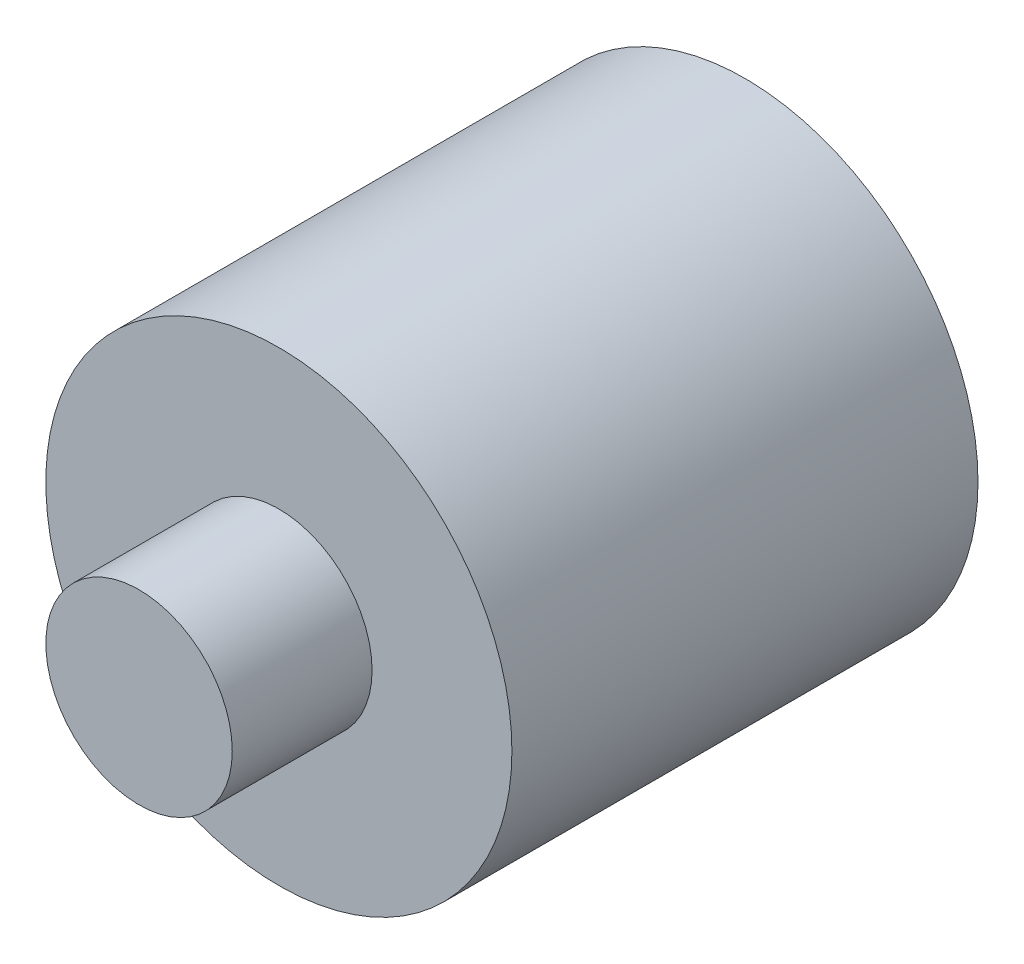
SolidWorks part; units mm, degrees
ref_plane "Front Plane" through (0, 0, 0) normal (0, 0, 1) x (1, 0, 0)
ref_plane "Top Plane" through (0, 0, 0) normal (0, 1, 0) x (1, 0, 0)
ref_plane "Right Plane" through (0, 0, 0) normal (1, 0, 0) x (0, 0, -1)
other "Configuration Table"
sketch "Sketch1" plane through (0, 0, 0) normal (0, 0, 1) x (1, 0, 0)
  circle A0 centre (0, 0) radius 2.5
  dimension "D1" = 5
extrude "Boss-Extrude1" add sketch "Sketch1" along normal blind 5
sketch "Sketch2" plane through (0, 0, 5) normal (0, 0, 1) x (1, 0, 0)
  circle A0 centre (0, 0) radius 1
  dimension "D1" = 2
extrude "Boss-Extrude2" add sketch "Sketch2" along normal blind 1.5
sketch "Sketch3" plane through (0, 0, 0) normal (0, 1, 0) x (1, 0, 0)
  line L0 (-2.4495, 0) -> (0, 0)
  line L2 (0, 0) -> (0, 3.7518) construction
  line L5 (0, 0) -> (0, -2)
  arc A1 (-2.4495, 0) -> (0, -2) centre (0, 0.5) ccw
  dimension "D2" = 0.5
  dimension "D1" = 5
revolve "Cut-Revolve1" cut sketch "Sketch3" angle 360 about L2
